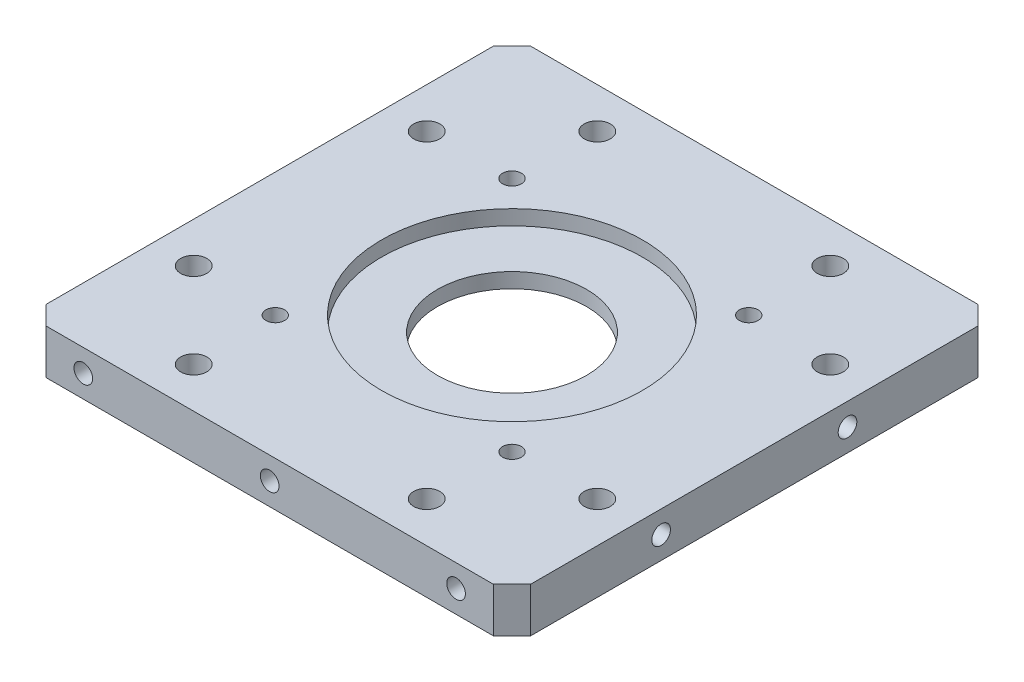
SolidWorks part; units mm, degrees
material "6061Al"
ref_plane "前视基准面" through (0, 0, 0) normal (0, 0, 1) x (1, 0, 0)
ref_plane "上视基准面" through (0, 0, 0) normal (0, 1, 0) x (1, 0, 0)
ref_plane "右视基准面" through (0, 0, 0) normal (1, 0, 0) x (0, 0, -1)
sketch "草图1" plane through (0, 0, 0) normal (0, 1, 0) x (1, 0, 0)
  line L1 (-65, -65) -> (65, -65)
  line L2 (-65, -65) -> (-65, 65)
  line L3 (-65, 65) -> (65, 65)
  line L4 (65, -65) -> (65, 65)
  line L5 (-65, -65) -> (65, 65) construction
  line L6 (-65, 65) -> (65, -65) construction
  point P0 (0, 0)
  dimension "D1" = 130
extrude "凸台-拉伸1" add sketch "草图1" along normal blind 12
sketch "草图2" plane through (0, 12, 0) normal (0, 1, 0) x (1, 0, 0)
  circle A0 centre (0, 0) radius 20
  dimension "D1" = 40
extrude "切除-拉伸1" cut sketch "草图2" against normal through all
hole_wizard "M6 间隙孔1" positions "草图3" profile "草图4" hole size "M6" standard "GB" end condition through all
sketch "草图3" plane through (0, 12, 0) normal (0, 1, 0) x (1, 0, 0)
  point P0 (31.25, 54.1266)
  point P3 (54.1266, 31.25)
  point P6 (54.1266, -31.25)
  point P9 (31.25, -54.1266)
  point P12 (-31.25, -54.1266)
  point P15 (-54.1266, -31.25)
  point P18 (-54.1266, 31.25)
  point P21 (-31.25, 54.1266)
sketch "草图4" plane through (31.25, 12, -54.1266) normal (1, 0, 0) x (0, 0, 1)
  line L0 (0, 0) -> (0, 12)
  line L1 (0, 12) -> (3.5, 12)
  line L2 (3.5, 12) -> (3.5, 0)
  line L5 (3.5, 0) -> (0, 0)
  line L11 (0, -6.35) -> (0, 107.95) construction
  dimension "通孔孔直径" = 7
  dimension "通孔孔深度" = 12
sketch "草图5" plane through (0, 12, 0) normal (0, 1, 0) x (1, 0, 0)
  circle A0 centre (0, 0) radius 35
  dimension "D1" = 70
extrude "切除-拉伸2" cut sketch "草图5" against normal blind 4
sketch "草图6" plane through (0, 0, 0) normal (0, -1, 0) x (1, 0, 0)
  circle A0 centre (0, 0) radius 45
  dimension "D1" = 90
extrude "切除-拉伸3" cut sketch "草图6" against normal blind 4
hole_wizard "M6 螺纹孔1" positions "草图7" profile "草图8" tap size "M6" standard "GB" end condition through all
sketch "草图7" plane through (0, 12, 0) normal (0, 1, 0) x (1, 0, 0)
  point P0 (-31.75, 31.75)
  point P3 (31.75, 31.75)
  point P6 (31.75, -31.75)
  point P9 (-31.75, -31.75)
sketch "草图8" plane through (-31.75, 12, -31.75) normal (1, 0, 0) x (0, 0, 1)
  line L0 (0, 0) -> (0, 12)
  line L1 (0, 12) -> (2.5, 12)
  line L2 (2.5, 12) -> (2.5, 0)
  line L5 (2.5, 0) -> (0, 0)
  line L11 (0, -6.35) -> (0, 107.95) construction
  dimension "通孔螺纹孔钻头直径" = 5
  dimension "通孔螺纹孔钻头深度" = 12
cosmetic thread "孔螺蚊线1" parameters "D2"=6
cosmetic thread "孔螺蚊线2" parameters "D2"=6
cosmetic thread "孔螺蚊线3" parameters "D2"=6
cosmetic thread "孔螺蚊线4" parameters "D2"=6
hole_wizard "M6 螺纹孔2" positions "草图9" profile "草图10" tap size "M6" standard "GB"
sketch "草图9" plane through (-65, 0, 0) normal (-1, 0, 0) x (0, 0, 1)
  line L0 (-65, 6) -> (65, 6) construction
  line L1 (-65, 12) -> (-65, 0) construction
  line L2 (65, 12) -> (65, 0) construction
  line L4 (0, -0.661) -> (0, 12) construction
  line L5 (-65, 12) -> (65, 12) construction
  point P0 (-25, 6)
  point P2 (25, 6)
  dimension "D1" = 50
sketch "草图10" plane through (-65, 6, -25) normal (0, 1, 0) x (0, 0, 1)
  line L0 (0, 0) -> (0, 16.5022)
  line L1 (0, 16.5022) -> (2.5, 15)
  line L2 (2.5, 15) -> (2.5, 0)
  line L5 (2.5, 0) -> (0, 0)
  line L10 (0, 16.5022) -> (-2.5, 15) construction
  line L11 (0, -6.35) -> (0, 107.95) construction
  dimension "螺纹孔钻头直径" = 5
  dimension "螺纹孔钻头深度" = 15
  dimension "导头角度" = 118
cosmetic thread "孔螺蚊线5" parameters "D1"=12, "D2"=6
cosmetic thread "孔螺蚊线6" parameters "D1"=12, "D2"=6
hole_wizard "M6 螺纹孔3" positions "草图11" profile "草图12" tap size "M6" standard "GB"
sketch "草图11" plane through (65, 0, 0) normal (1, 0, 0) x (0, 0, -1)
  point P0 (-25, 6)
  point P3 (25, 6)
sketch "草图12" plane through (65, 6, 25) normal (0, 1, 0) x (0, 0, -1)
  line L0 (0, 0) -> (0, 16.5022)
  line L1 (0, 16.5022) -> (2.5, 15)
  line L2 (2.5, 15) -> (2.5, 0)
  line L5 (2.5, 0) -> (0, 0)
  line L10 (0, 16.5022) -> (-2.5, 15) construction
  line L11 (0, -6.35) -> (0, 107.95) construction
  dimension "螺纹孔钻头直径" = 5
  dimension "螺纹孔钻头深度" = 15
  dimension "导头角度" = 118
cosmetic thread "孔螺蚊线7" parameters "D1"=12, "D2"=6
cosmetic thread "孔螺蚊线8" parameters "D1"=12, "D2"=6
hole_wizard "M6 螺纹孔4" positions "草图13" profile "草图14" tap size "M6" standard "GB"
sketch "草图13" plane through (0, 0, 65) normal (0, 0, 1) x (1, 0, 0)
  line L0 (-65, 6) -> (65, 6) construction
  line L1 (-65, 12) -> (-65, 0) construction
  line L2 (65, 12) -> (65, 0) construction
  line L4 (0, 0) -> (0, 12) construction
  line L5 (-65, 12) -> (65, 12) construction
  point P0 (-50, 6)
  point P2 (50, 6)
  point P18 (0, 6)
  dimension "D1" = 100
sketch "草图14" plane through (-50, 6, 65) normal (1, 0, 0) x (0, -1, 0)
  line L0 (0, 0) -> (0, 16.5022)
  line L1 (0, 16.5022) -> (2.5, 15)
  line L2 (2.5, 15) -> (2.5, 0)
  line L5 (2.5, 0) -> (0, 0)
  line L10 (0, 16.5022) -> (-2.5, 15) construction
  line L11 (0, -6.35) -> (0, 107.95) construction
  dimension "螺纹孔钻头直径" = 5
  dimension "螺纹孔钻头深度" = 15
  dimension "导头角度" = 118
cosmetic thread "孔螺蚊线9" parameters "D1"=12, "D2"=6
cosmetic thread "孔螺蚊线10" parameters "D1"=12, "D2"=6
cosmetic thread "孔螺蚊线13" parameters "D1"=12, "D2"=6
hole_wizard "M6 螺纹孔5" positions "草图15" profile "草图17" tap size "M6" standard "ISO"
sketch "草图15" plane through (0, 0, -65) normal (0, 0, -1) x (-1, 0, 0)
  point P0 (-50, 6)
  point P3 (50, 6)
  point P6 (0, 6)
sketch "草图17" plane through (50, 6, -65) normal (1, 0, 0) x (0, 1, 0)
  line L0 (0, 0) -> (0, 16.5022)
  line L1 (0, 16.5022) -> (2.5, 15)
  line L2 (2.5, 15) -> (2.5, 0)
  line L5 (2.5, 0) -> (0, 0)
  line L10 (0, 16.5022) -> (-2.5, 15) construction
  line L11 (0, -6.35) -> (0, 107.95) construction
  dimension "螺纹孔钻头直径" = 5
  dimension "螺纹孔钻头深度" = 15
  dimension "导头角度" = 118
cosmetic thread "孔螺蚊线11" parameters "D1"=12, "D2"=6
cosmetic thread "孔螺蚊线12" parameters "D1"=12, "D2"=6
cosmetic thread "孔螺蚊线14" parameters "D1"=12, "D2"=6
chamfer "倒角1" distance 5 angle 45 4 edges at (-65, 6, 65) (65, 6, 65) (65, 6, -65) (-65, 6, -65)
